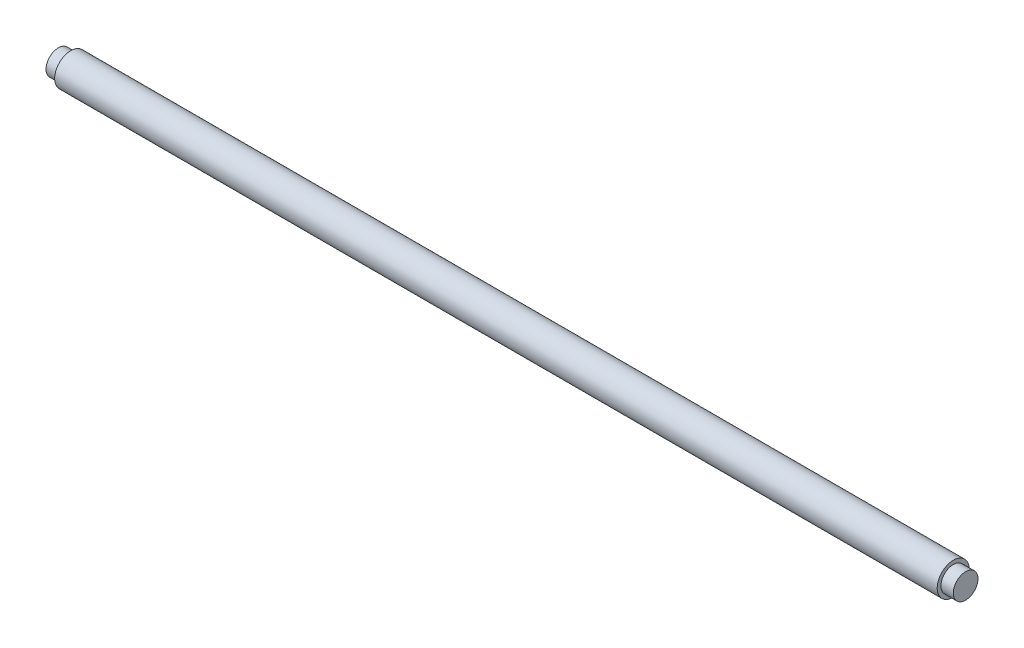
from build123d import *

# Parameters (mm, degrees)
SKETCH1_R           = 6.5
BOSS_EXTRUDE1_DEPTH = 178.5
SKETCH2_R           = 5
BOSS_EXTRUDE2_DEPTH = 5
BOSS_EXTRUDE3_START = 5
SKETCH3_R           = 5
BOSS_EXTRUDE3_DEPTH = 5


with BuildPart() as part:
    # Sketch1 → Boss-Extrude1 (new, symmetric)
    with BuildSketch(Plane(origin=(0, 0, 0), x_dir=(0, 0, -1), z_dir=(1, 0, 0))):
        Circle(SKETCH1_R)
    extrude(amount=BOSS_EXTRUDE1_DEPTH, both=True)

    # Sketch2 → Boss-Extrude2 (add)
    with BuildSketch(Plane(origin=(178.5, 0, 0), x_dir=(0, 0, -1), z_dir=(1, 0, 0))):
        Circle(SKETCH2_R)
    extrude(amount=BOSS_EXTRUDE2_DEPTH)

    # Sketch3 → Boss-Extrude3 (add)
    with BuildSketch(Plane.ZY.offset(178.5).offset(BOSS_EXTRUDE3_START)):
        with Locations(Location((0, 0, 0), (0, 0, 180))):
            Circle(SKETCH3_R)
    extrude(amount=-BOSS_EXTRUDE3_DEPTH)


solid = part.part
